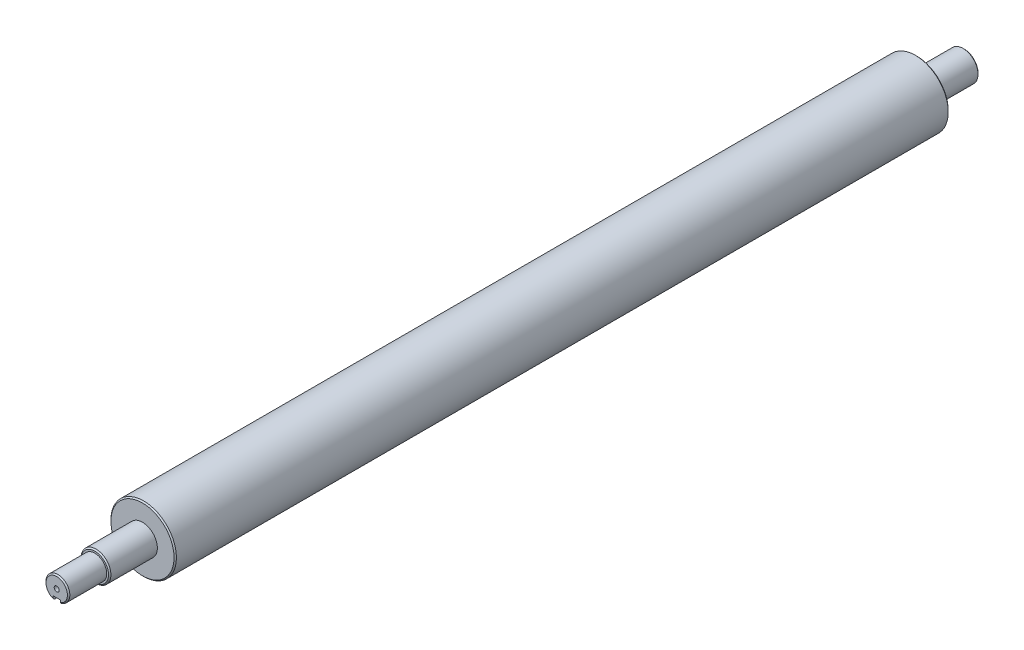
SolidWorks part; units mm, degrees
ref_plane "Front Plane" through (0, 0, 0) normal (0, 0, 1) x (1, 0, 0)
ref_plane "Top Plane" through (0, 0, 0) normal (0, 1, 0) x (1, 0, 0)
ref_plane "Right Plane" through (0, 0, 0) normal (1, 0, 0) x (0, 0, -1)
sketch "Sketch1" plane through (0, 0, 0) normal (0, 0, 1) x (1, 0, 0)
  circle A0 centre (0, 0) radius 27.5
  dimension "D1" = 55
extrude "Boss-Extrude1" add sketch "Sketch1" along normal mid plane 650
sketch "Sketch2" plane through (0, 0, 325) normal (0, 0, 1) x (1, 0, 0)
  circle A0 centre (0, 0) radius 12.5
  dimension "D1" = 25
extrude "Boss-Extrude2" add sketch "Sketch2" along normal blind 40
mirror "Mirror1" about plane through (0, 0, 0) normal (0, 0, 1) of "Boss-Extrude2"
chamfer "Chamfer1" distance 1 angle 45 4 edges at (12.5, 0, -365) (27.5, 0, -325) (12.5, 0, 365) (27.5, 0, 325)
sketch "Sketch3" plane through (0, 0, 365) normal (0, 0, 1) x (1, 0, 0)
  circle A0 centre (0, 0) radius 10
  dimension "D1" = 20
extrude "Boss-Extrude3" add sketch "Sketch3" along normal blind 32
chamfer "Chamfer2" distance 1 angle 45 1 edges at (10, 0, 397)
sketch "Sketch4" plane through (0, 0, 0) normal (0, 1, 0) x (1, 0, 0)
  line L0 (0, -424.5) -> (0, -369.5) construction
  line L1 (-9, -397) -> (9, -397) construction
  line L2 (-3, -424.5) -> (-3, -369.5)
  line L3 (3, -424.5) -> (3, -369.5)
  arc A0 (-3, -424.5) -> (3, -424.5) centre (0, -424.5) ccw
  arc A1 (3, -369.5) -> (-3, -369.5) centre (0, -369.5) ccw
  point P5 (0, -397)
  dimension "D2" = 3
  dimension "D1" = 55
extrude "Cut-Extrude1" cut sketch "Sketch4" against normal blind 10 from offset 6.5 offset against normal yes
hole_wizard "M5 Tapped Hole1" positions "Sketch5" profile "Sketch6" tap size "M5" standard "GB"
sketch "Sketch5" plane through (0, 0, 397) normal (0, 0, 1) x (1, 0, 0)
  point P0 (0, 0)
sketch "Sketch6" plane through (0, 0, 397) normal (1, 0, 0) x (0, -1, 0)
  line L0 (0, 0) -> (0, 13.6618)
  line L1 (0, 13.6618) -> (2.1, 12.4)
  line L2 (2.1, 12.4) -> (2.1, 0)
  line L5 (2.1, 0) -> (0, 0)
  line L10 (0, 13.6618) -> (-2.1, 12.4) construction
  line L11 (0, -6.35) -> (0, 107.95) construction
  dimension "螺纹孔钻头直径" = 4.2
  dimension "螺纹孔钻头深度" = 12.4
  dimension "导头角度" = 118
cosmetic thread "Cosmetic Thread1" parameters "D1"=10, "D2"=5
